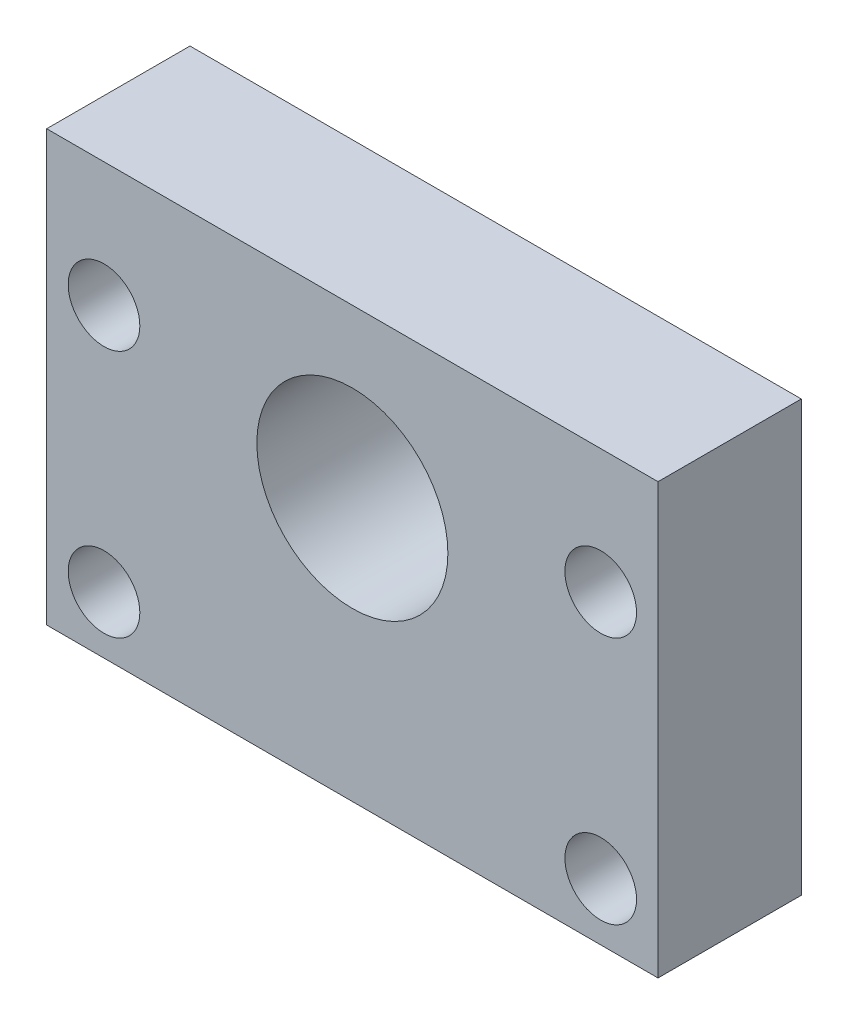
SolidWorks part; units mm, degrees
material "Q235A"
ref_plane "Front Plane" through (0, 0, 0) normal (0, 0, 1) x (1, 0, 0)
ref_plane "Top Plane" through (0, 0, 0) normal (0, 1, 0) x (1, 0, 0)
ref_plane "Right Plane" through (0, 0, 0) normal (1, 0, 0) x (0, 0, -1)
sketch "Sketch1" plane through (0, 0, 0) normal (0, 0, 1) x (1, 0, 0)
  line L1 (64, -45) -> (-64, -45)
  line L2 (64, -45) -> (64, 45)
  line L3 (64, 45) -> (-64, 45)
  line L4 (-64, -45) -> (-64, 45)
  line L5 (64, -45) -> (-64, 45) construction
  line L6 (64, 45) -> (-64, -45) construction
  point P0 (0, 0)
  dimension "D1" = 128
  dimension "D2" = 90
extrude "Boss-Extrude1" add sketch "Sketch1" along normal blind 30
sketch "Sketch4" plane through (0, 0, 30) normal (0, 0, 1) x (1, 0, 0)
  line L0 (64, 45) -> (-64, 45) construction
  circle A0 centre (0, 10) radius 20
  dimension "D2" = 40
  dimension "D1" = 35
extrude "Cut-Extrude3" cut sketch "Sketch4" against normal through all
hole_wizard "Ø15.0 (15) Diameter Hole1" positions "Sketch5" profile "Sketch7" hole size "Ø15.0" standard "GB"
sketch "Sketch5" plane through (0, 0, 30) normal (0, 0, 1) x (1, 0, 0)
  line L0 (0, 45) -> (0, 0) construction
  line L1 (64, 45) -> (-64, 45) construction
  line L3 (-64, -45) -> (64, -45) construction
  line L4 (-64, 45) -> (-64, -45) construction
  point P0 (-52, 19)
  point P2 (-52, -33)
  point P12 (52, -33)
  point P13 (52, 19)
  dimension "D1" = 26
  dimension "D2" = 12
  dimension "D3" = 12
sketch "Sketch7" plane through (-52, 19, 30) normal (1, 0, 0) x (0, -1, 0)
  line L0 (0, 0) -> (0, 46.5065)
  line L1 (0, 46.5065) -> (7.5, 42)
  line L2 (7.5, 42) -> (7.5, 0)
  line L5 (7.5, 0) -> (0, 0)
  line L10 (0, 46.5065) -> (-7.5, 42) construction
  line L11 (0, -6.35) -> (0, 107.95) construction
  dimension "孔直径" = 15
  dimension "孔深度" = 42
  dimension "导头角度" = 118
